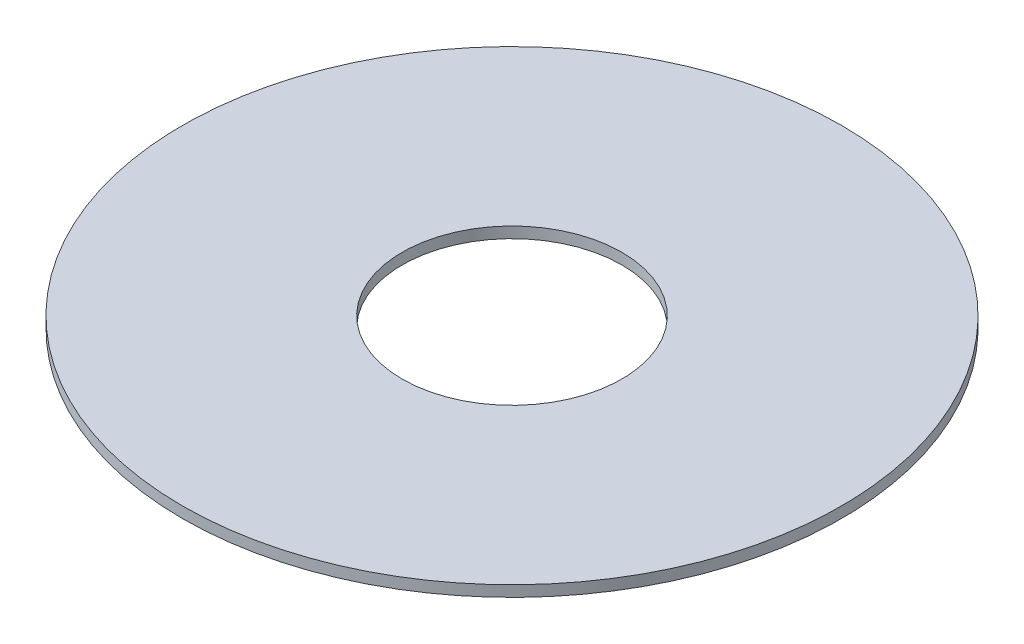
from build123d import *

# Parameters (mm, degrees)
SKETCH1_R           = 60
SKETCH1_R_2         = 20
BOSS_EXTRUDE1_DEPTH = 2


with BuildPart() as part:
    # Sketch1 → Boss-Extrude1 (new body)
    with BuildSketch(Plane(origin=(0, 0, 0), x_dir=(1, 0, 0), z_dir=(0, 1, 0))):
        with Locations(Location((0, 0, 0), (0, 0, 270))):
            Circle(SKETCH1_R)
        with Locations(Location((0, 0, 0), (0, 0, 270))):
            Circle(SKETCH1_R_2, mode=Mode.SUBTRACT)
    extrude(amount=BOSS_EXTRUDE1_DEPTH)


solid = part.part
